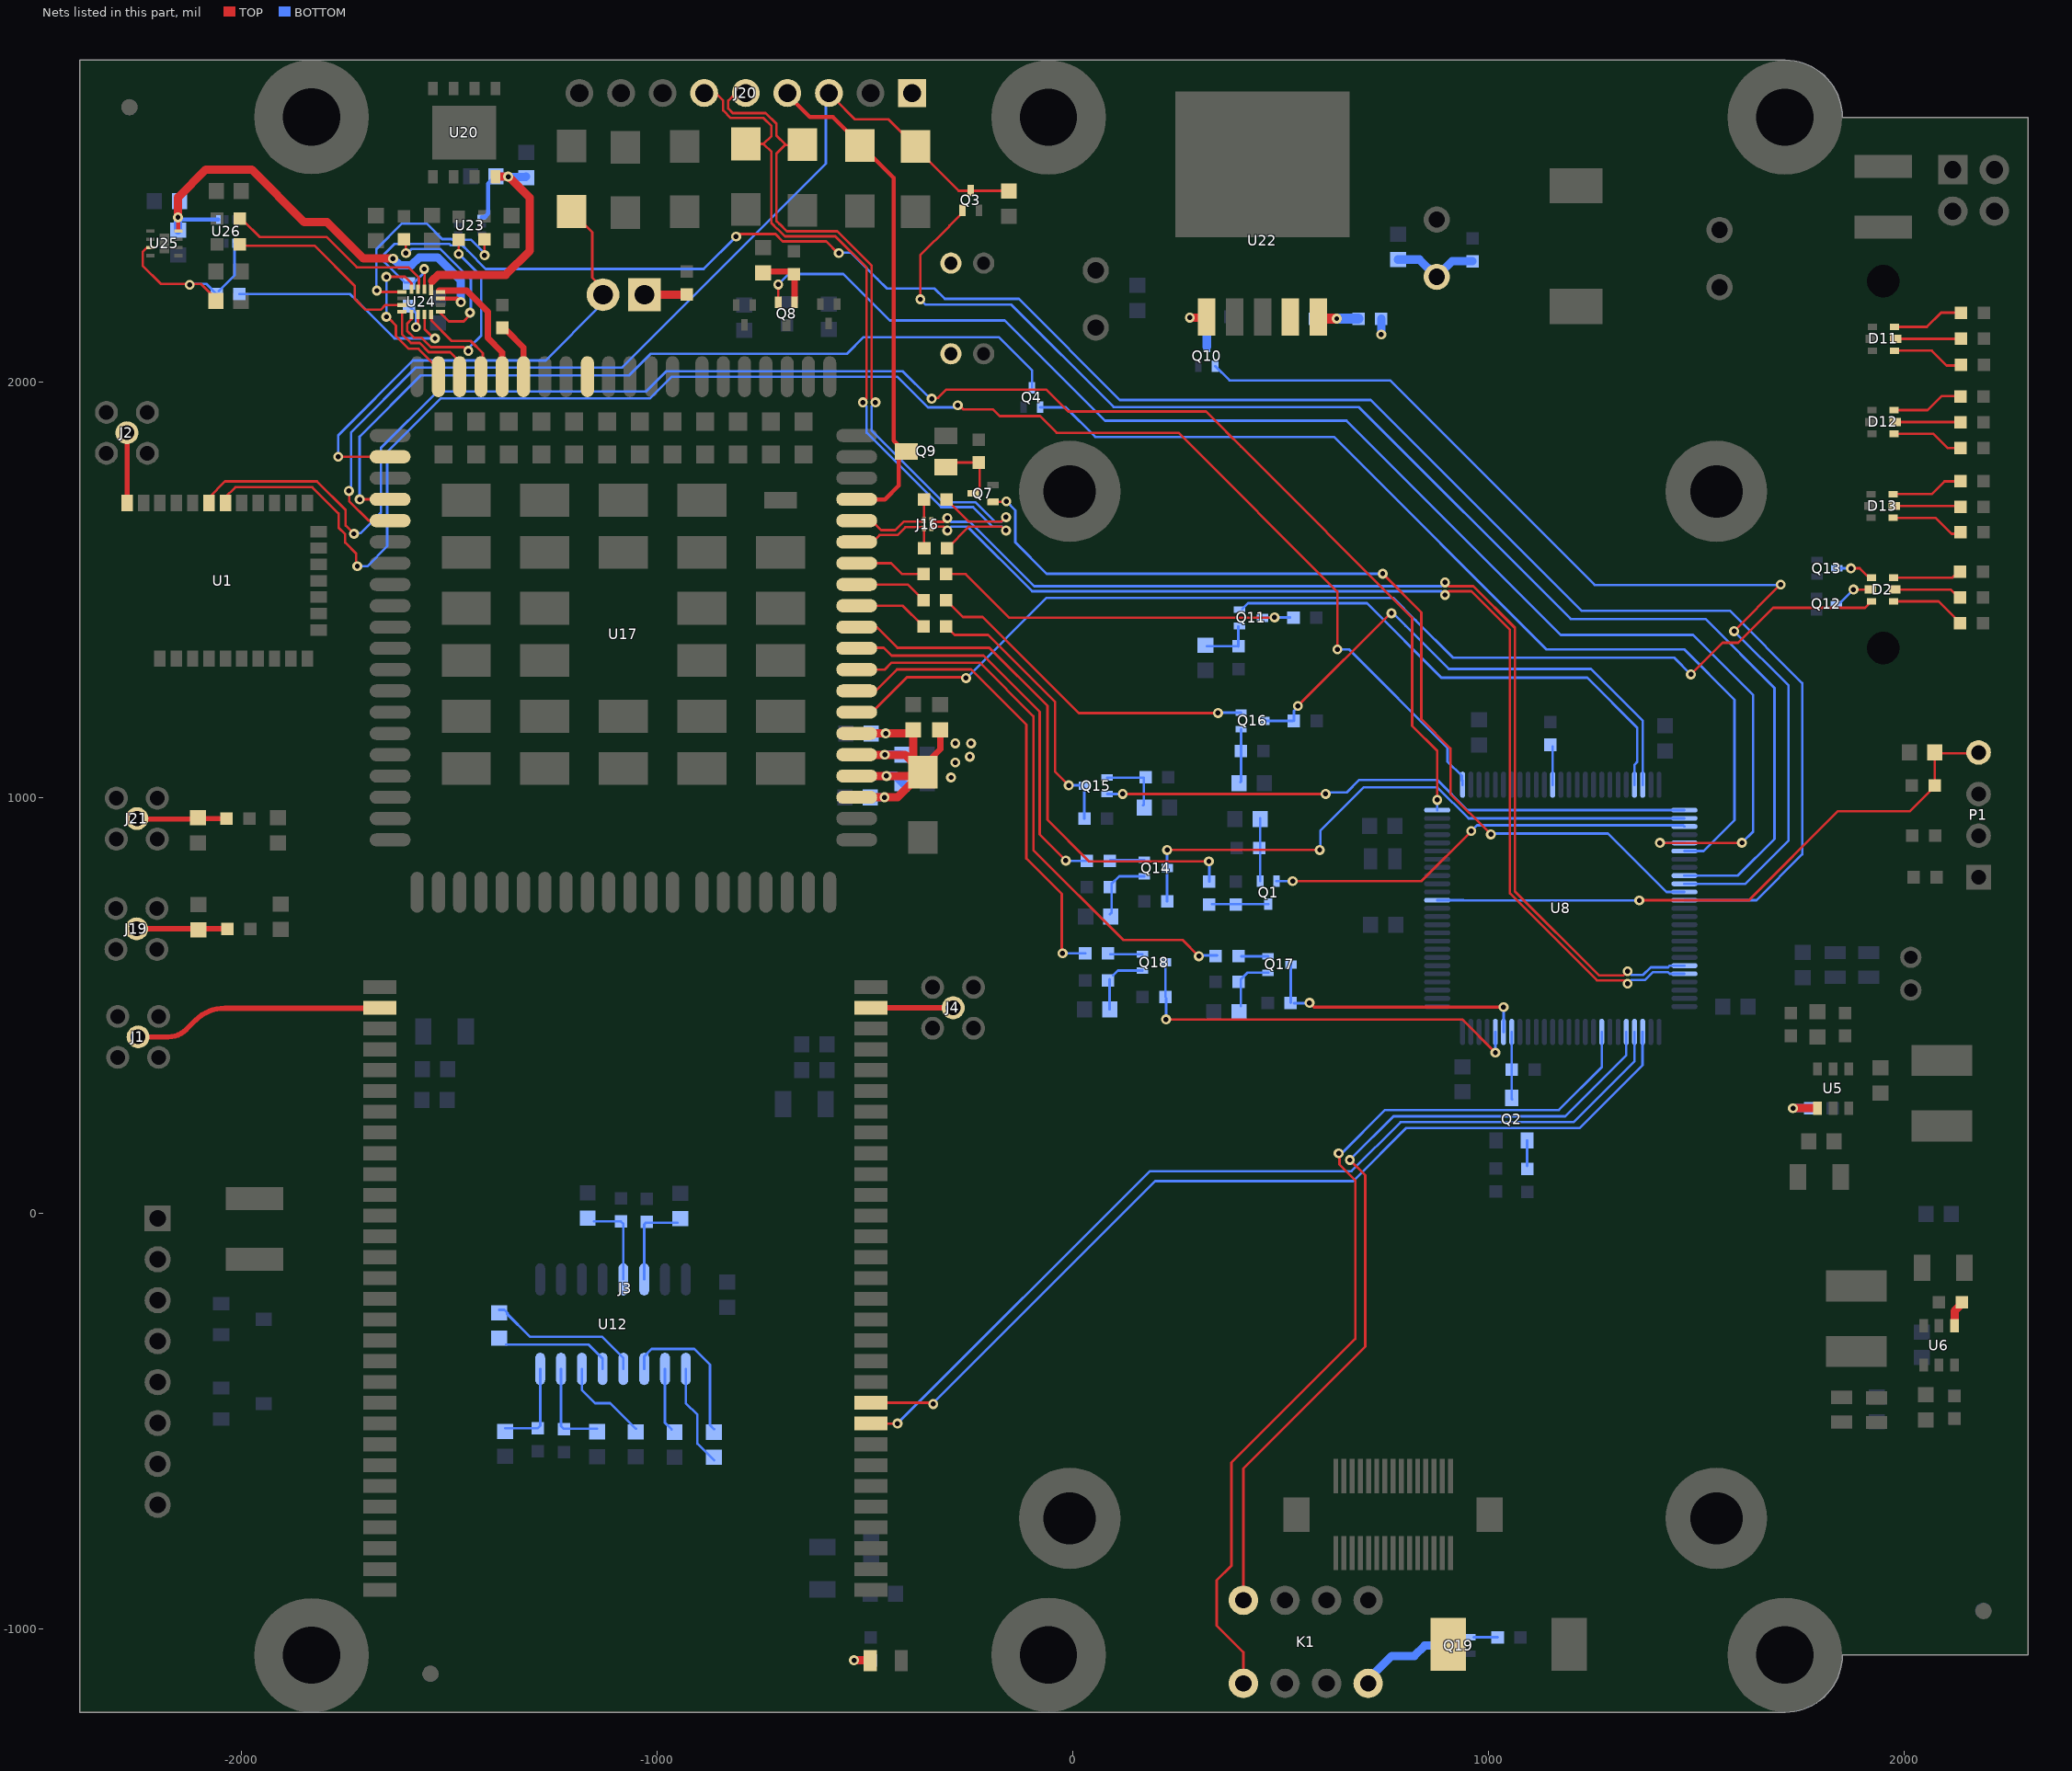
[diagram p0: the nets of this part, all layers, seen from the top]
# Altium PCB MISC84456.PcbDoc (part 4 of 5)
Units mil, origin at the board's own origin, x right, y up, seen from the top; angles counter-clockwise.
Board outline 4685.04 x 3973.82 mil, 4 copper layers (TOP, GND, POWER, BOTTOM), stack 38.4 mil thick; 219 components, 175 nets, 938 pads, 792 vias.

## Via types
v1: diameter 24, hole 12, TOP to BOTTOM, 400 vias
v2: diameter 24, hole 12, TOP to BOTTOM, tented both sides, 388 vias
v3: diameter 40, hole 20, TOP to BOTTOM, 4 vias

## Nets (pads, with @x,y where several pads share a name; then routed paths per layer and width w, separated by ;. In a path a pad name is that pad's centre, name@x,y a point inside that pad or via, vN(x,y) a via of type N, cw(c..) or ccw(c..) an arc to the next point about the centre after c; other vN are vias at no path point) (continued)
NetC52_1: C52.1 R24.2 U25.3 U26.4 | length 451.1
  TOP w6: U25.3@-2218.15,2323.71 -2226.29,2323.71 -2237,2313 -2237,2280 -2193,2236 -2097,2236 C52.1@-2071,2210
  BOTTOM w6: v2@-2118,2236 -2083.74,2236 R24.2@-2059.18,2211.44 ; R24.2@-2054,2219 -2016,2257 -2016,2313 U26.4@-2016,2334.11
  other v2: -2124,2234
NetC57_2: C57.2 Q1.2 R39.1 | length 151.1
  BOTTOM w6: Q1.2@450.32,799.56 C57.2@450.32,949 C57.2@450.32,950.69
NetC58_1: C58.1 Q8.2 R31.2 | length 144.2
  TOP w6: R31.2@-671,2263 R31.2@-669.31,2264.69
  TOP w15: C58.1@-740,2266 -675,2266 -669.31,2260.32 Q8.2@-669.31,2191.56
NetC59_2: C59.2 Q11.2 R40.1 | length 123.8
  BOTTOM w6: C59.2@322.5,1364.5 R40.1@397.69,1364.5 ; R40.1@397.69,1364 R40.1@397.69,1364.5 ; Q11.2@397.69,1412.32 R40.1@397.69,1364.5 ; R40.1@398,1364.5 R40.1@397.69,1364.5
NetC60_2: C60.2 Q15.2 R43.1 | length 155.5
  BOTTOM w6: Q15.2@82.56,1048.69 170.69,1048.69 170.69,983.69 C60.2@169,982
NetC61_1: C61.1 Q14.2 R48.2 | length 160.7
  BOTTOM w6: C61.1@89,720 93,724 93,793 111.32,811.32 Q14.2@171.44,811.32
NetC62_1: C62.1 Q16.2 R51.2 | length 127.9
  BOTTOM w6: C62.1@403,1038 404.44,1039.44 Q16.2@404.44,1165.32
NetC63_1: C63.1 Q17.2 R54.2 | length 136.8
  BOTTOM w6: C63.1@404,499 404,564 419.32,579.32 Q17.2@469.44,579.32
NetC64_1: C64.1 Q18.2 R56.2 | length 147.8
  BOTTOM w6: C64.1@88.32,491 R56.2@88.32,563.69 ; R56.2@97,573 108.32,584.32 Q18.2@167.44,584.32
NetC87_1: C87.1 U12.3 | length 370.4
  BOTTOM w6: U12.3@-1031,-373.59 -1031,-343.8 -1013,-325.8 -910.2,-325.8 -873,-363 -873,-508.6 C87.1@-863,-518.6
NetC87_2: C87.2 U12.1 | length 257.6
  BOTTOM w6: -931,-444.6 -931,-435 ; U12.1@-931,-373.59 -931,-435 ; C87.2@-863,-593.4 -903.1,-553.3 -903.1,-483.9 -931,-456 -931,-435
NetC92_1: C92.1 U12.2 | length 226.6
  BOTTOM w6: -981,-495.6 -981,-421 ; U12.2@-981,-373.59 -981,-421 ; C92.1@-965,-519 -981,-503 -981,-421
NetC93_1: C93.1 U12.5 | length 270.7
  BOTTOM w6: C93.1@-1363,-315 -1165,-315 -1131,-349 U12.5@-1131,-373.59
NetC93_2: C93.2 U12.4 | length 373.7
  BOTTOM w6: C93.2@-1380,-231.6 -1367.4,-231.6 -1359.5,-239.5 ; C93.2@-1361,-241 -1306,-296 -1133,-296 -1081,-348 U12.4@-1081,-373.59
NetC94_2: C94.2 R59.2 U12.14 | length 213.9
  BOTTOM w6: U12.14@-1031,-158.2 -1031,-26 -1027,-22 C94.2@-951,-22
NetC95_2: C95.2 R60.2 U12.13 | length 206.7
  BOTTOM w6: C95.2@-1152,-19 -1087,-19 -1081,-25 U12.13@-1081,-158.2
NetC96_1: C96.1 U12.6 | length 219.2
  BOTTOM w6: U12.6@-1181,-373.59 -1181,-424 -1149,-456 -1112.6,-456 C96.1@-1051,-517.6
NetC97_2: C97.2 J19.1 R62.2 | length 207.5
  TOP w12.5: J19.1@-2240,686 -2240,685 R62.2@-2033.5,685
NetC99_1: C99.1 R63.2 U12.8 | length 223.3
  BOTTOM w6: C99.1@-1365,-516.5 -1287.1,-516.5 -1281,-510.4 U12.8@-1281,-373.59
NetC100_1: C100.1 R61.2 U12.7 | length 227.3
  BOTTOM w6: U12.7@-1231,-373.59 -1231,-511.4 -1224.9,-517.5 C100.1@-1144,-517.5
NetC102_2: C102.2 J21.1 R64.2 | length 208.5
  TOP w12.5: J21.1@-2243,949 -2101,949 -2101,950 R64.2@-2035.5,950
NetD1_1: D1.1 K1.8 Q19.3 | length 214.9
  BOTTOM w20: K1.8@716,-1115 767,-1064 821,-1064 846,-1039 Q19.3@899.44,-1039
NetD2_2: D2.2 R1.2 | length 172.3
  TOP w6: D2.2@1973.57,1472.46 2081.54,1472.46 R1.2@2127,1427
NetD2_3: D2.3 Q12.3 | length 84.3
  TOP w6: v1(1877,1501) D2.3@1917.47,1501
  BOTTOM w6: Q12.3@1846,1470 v1(1877,1501)
NetD2_4: D2.4 R2.2 | length 151.4
  TOP w6: D2.4@1976.53,1501 2111,1501 R2.2@2123,1489
NetD2_5: D2.5 Q13.3 | length 85.1
  TOP w6: v1(1871,1552) 1892,1552 D2.5@1913,1531
  BOTTOM w6: Q13.3@1836.62,1552 v1(1871,1552)
NetD2_6: D2.6 R3.2 | length 158.2
  TOP w6: D2.6@1973.57,1529.54 2115.54,1529.54 R3.2@2127,1541
NetD7_1: D7.1 R18.2 | length 79.2
  TOP w20: v2(-526.5,-1074.5) -488.5,-1074.5 D7.1@-488,-1074
  BOTTOM w20: v2(-526.5,-1074.5) R18.2@-486,-1074.5
NetD11_2: D11.2 R75.2 | length 175.1
  TOP w6: D11.2@1975.57,2075.46 2065.54,2075.46 2101,2040 R75.2@2136,2040
NetD11_4: D11.4 R76.2 | length 161.5
  TOP w6: D11.4@1978.53,2104 R76.2@2135.5,2104 R76.2@2140,2104
NetD11_6: D11.6 R81.2 | length 173.7
  TOP w6: D11.6@1975.57,2132.54 2053.54,2132.54 2088,2167 R81.2@2135,2167
NetD12_2: D12.2 R82.2 | length 172.7
  TOP w6: D12.2@1974.57,1875.46 2069.54,1875.46 2104,1841 R82.2@2133,1841
NetD12_4: D12.4 R86.2 | length 151.5
  TOP w6: D12.4@1977.53,1904 R86.2@2129,1904
NetD12_6: D12.6 R92.2 | length 170.3
  TOP w6: D12.6@1974.57,1932.54 2055.54,1932.54 2089,1966 R92.2@2131,1966
NetD13_2: D13.2 R85.2 | length 180.4
  TOP w6: D13.2@1972.57,1673.46 2074.54,1673.46 2113,1635 R85.2@2137,1635
NetD13_4: D13.4 R91.2 | length 157.5
  TOP w6: D13.4@1975.53,1702 R91.2@2133,1702
NetD13_6: D13.6 R94.2 | length 173
  TOP w6: D13.6@1972.57,1730.54 2065.54,1730.54 2096,1761 R94.2@2133,1761
NetJ1_1: J1.1 J3.2 | length 614
  TOP w12.5: J1.1@-2248,425 -2175.46,425 ccw(c-2175.46,486.46) -2132,443 -2110.29,464.71 cw(c-2039.58,394) -2039.58,494 J3.2@-1673,494 ; J3.2@-1678.58,495 J3.2@-1666.55,495 ccw(c-1671.38,490.17) J3.2@-1671.38,497
NetJ2_1: J2.1 U1.29 | length 154.3
  TOP w12.5: U1.29@-2274.31,1709.01 J2.1@-2274.31,1863.32
NetJ3_59: J3.59 J4.1 | length 175
  TOP w12.5: J3.59@-461,497 -461,495 J4.1@-288,495
NetJ16_2: J16.2 R33.2 U17.69 | length 221.7
  TOP w6: U17.69@-519.98,1615.44 -481.56,1615.44 -465,1632 -422,1632 -403,1651 J16.2@-360,1651 ; R33.2@-357.86,1601.14 J16.2@-357.86,1648.16
NetJ16_3: J16.3 R34.2 U17.70 | length 219.7
  TOP w6: U17.70@-519.98,1666.62 -483.62,1666.62 -461,1644 -426.97,1644 -406.92,1664.05 J16.3@-361,1664.05 ; J16.3@-357.86,1667.84 R34.2@-357.86,1710.86
NetJ26_1: J26.1 R77.2 | length 77.5
  TOP w20: J26.1@-1006.5,2210.5 R77.2@-929,2210.5
NetQ1_3: Q1.3 R26.1 R41.2 | length 135.4
  BOTTOM w6: R26.1@334.56,744.44 Q1.3@470,744.44
NetQ2_1: Q2.1 R37.1 | length 61.2
  BOTTOM w6: R37.1@1092.4,114.6 Q2.1@1092.4,175.82
NetQ2_3: Q2.3 R36.2 U8.94 | length 162.2
  BOTTOM w6: U8.94@1055.24,436.88 1055.24,275.76 Q2.3@1056,275
NetQ7_3: Q7.3 Q9.1 R29.2 | length 172
  TOP w6: Q9.1@-298,1806 -297.62,1806.38 R29.2@-222,1806.38 ; Q7.3@-230,1737 -224,1743 -224,1781 ; -224,1750.62 -224,1781 ; R29.2@-224,1800 -224,1781
NetQ10_3: Q10.3 R65.1 U22.1 | length 132.4
  TOP w20: v2(281,2155) U22.1@303,2155
  BOTTOM w20: v2(281,2155) 322,2155 Q10.3@322,2085.62
NetQ11_3: Q11.3 R32.1 R44.2 | length 894
  TOP w6: R32.1@-304.5,1538 -258,1538 -153,1433 v1@480,1433 ; v1@482.5,1430.5 v1@485,1433
  BOTTOM w6: Q11.3@455.56,1433 v1@481,1433 ; v1(485,1434) R44.2@522,1434
NetQ14_1: Q14.1 R47.1 | length 81.8
  BOTTOM w6: R47.1@89.69,850.69 Q14.1@171.44,850.69
NetQ15_3: Q15.3 R27.1 R45.2 | length 665.1
  TOP w6: R27.1@-304.5,1412 -284.5,1392 -204,1392 -43,1231 -43,1063 v1(-10,1030)
  BOTTOM w6: v1(-10,1030) 24,1030 Q15.3@24,1024.5 ; R45.2@27.5,950 Q15.3@27.5,1024.5
NetQ16_1: Q16.1 R28.1 | length 815.9
  TOP w6: R28.1@-304.5,1475 -264.5,1435 -217,1435 14,1204 v1(349,1204)
  BOTTOM w6: v1(349,1204) v1@350,1205 ; v1@355.69,1204.69 Q16.1@404.44,1204.69
NetQ17_1: Q17.1 R50.1 | length 64.8
  BOTTOM w6: R50.1@404.69,618.69 Q17.1@469.44,618.69
NetQ18_1: Q18.1 R52.1 | length 77.8
  BOTTOM w6: R52.1@89.69,623.69 Q18.1@167.44,623.69
NetQ19_2: Q19.2 R57.1 | length 57.5
  BOTTOM w6: Q19.2@964,-1019 R57.1@1021.5,-1019
NetR12_1: R12.1 U5.4 | length 103
  TOP w20: v1(1731.6,253.4) U5.4@1790.6,253.4
  BOTTOM w20: v1(1731.6,253.4) R12.1@1775.6,253.4
NetR19_1: R19.1 U6.4 | length 57.2
  TOP w20: U6.4@2120.4,-269.76 2120.4,-234.6 R19.1@2136,-219
NetR22_2: R22.2 U24.10 | length 83.5
  TOP w6: v2(-1580,2132) -1574.87,2137.13 U24.10@-1574.87,2162.44
  BOTTOM w6: R22.2@-1592,2178 -1580,2166 v2(-1580,2132)
NetR26_2: R26.2 U17.65 | length 1283.5
  TOP w6: U17.65@-519.98,1410.72 -471.72,1410.72 -422,1361 -346,1361 -201,1361 -61,1221 -61,947 39,847 v1(327,847)
  BOTTOM w6: R26.2@328,798.5 v1@328,841
NetR27_2: R27.2 U17.66 | length 176
  TOP w6: U17.66@-519.98,1461.9 -408.9,1461.9 R27.2@-363,1416
NetR28_2: R28.2 U17.67 | length 166.8
  TOP w6: U17.67@-519.98,1513.08 -397.08,1513.08 R28.2@-366,1482
NetR32_2: R32.2 U17.68 | length 169.9
  TOP w6: U17.68@-519.98,1564.26 -437.26,1564.26 -411,1538 R32.2@-361,1538
NetR47_2: R47.2 U17.64 | length 933.4
  TOP w6: U17.64@-519.98,1359.54 U17.64@-500,1359.54 ; U17.64@-500,1359 U17.64@-487,1359 ; U17.64@-487,1361 -455,1361 -436,1342 -215,1342 -80,1207 -80,912 v1(-17,849)
  BOTTOM w6: v1@-12,848 R47.2@33.5,848
NetR50_2: R50.2 U17.63 | length 1355.8
  TOP w6: U17.63@-519.98,1308.35 -452.65,1308.35 -436,1325 -224,1325 -95,1196 -95,874 121,658 264,658 v1(303,619)
  BOTTOM w6: v1(303,619) 305,621 R50.2@347,621
NetR52_2: R52.2 U17.62 | length 1121.2
  TOP w6: U17.62@-519.98,1257.17 -474.83,1257.17 -423,1309 -245,1309 -112,1176 -112,854 -27,769 v1@-27,629
  BOTTOM w6: v1(-25,626) R52.2@29.5,626
NetR66_1: R66.1 R68.2 U22.5 | length 143.2
  TOP w25: U22.5@588,2153 588.5,2152.5 v1(634.5,2152.5)
  BOTTOM w25: R68.2@590,2152.5 v1(634.5,2152.5) R66.1@686.5,2152.5
NRST: C1.2 P1.4 R35.1 U8.14 | length 1488.2
  TOP w6: v1@1356,756 1358.19,753.81 1557,753.81 1625.81,753.81 1840,968 2013,968 R35.1@2071,1026 ; R35.1@2072.5,1030 2072.5,1103.5 2076,1107 P1.4@2172,1107
  BOTTOM w6: U8.14@876.11,753.81 938.81,753.81 ; 939.63,753 v1(1362,753)
ON/OFF_MCU: Q3.1 U8.59 | length 3302.4
  TOP w6: v1@-367,2210 -367,2305 -297,2375 -297,2376 -266,2407 Q3.1@-266,2413.38
  BOTTOM w6: v1(-367,2199) -354,2186 -148,2186 98,1940 687,1940 1197,1430 1521,1430 1687,1264 1687,901 1598.86,812.86 U8.59@1470.59,812.86
PB2_BOOT1: R4.2 U8.37 | length 92
  BOTTOM w6: U8.37@1153.67,1031.36 R4.2@1153.67,1123.33
PWRKEY: C32.1 D17.2 J20.3 Q3.3 U17.21 | length 2330.4
  TOP w6: v2@-1740,1733 -1740,1712.91 -1693.71,1666.62 U17.21@-1642.02,1666.62 ; J20.3@-573,2681 -524,2632 -443.26,2632 D17.2@-378,2566.74 ; D17.2@-351,2536 -298,2483 -275,2460 -159,2460 C32.1@-157,2462
  BOTTOM w6: v2@-1743,1735 v2@-1741,1737 ; v2@-1741,1735 v2@-1741,1737 ; v2(-1741,1738) v2@-1741,1737 ; J20.3@-594,2690 -594,2525 -1084,2035 -1580,2035 -1736.2,1878.8 -1736.2,1797 -1736.2,1756 -1736.2,1741.8 v2@-1741,1737
RESET_MCU: Q4.1 U8.56 | length 2402.4
  BOTTOM w6: Q4.1@-79,1939.38 -17.38,1939.38 54,1868 573,1868 628,1868 1139,1357 1470,1357 1591,1236 1591,946 1516.92,871.92 U8.56@1470.59,871.92
RESET_N: Q4.3 U17.20 | length 2014.6
  TOP w6: v2(-1715.2,1717.8) U17.20@-1642.02,1717.8
  BOTTOM w6: v2(-1715.2,1717.8) -1715.2,1868.8 -1568,2016 -1067,2016 -1015,2068 -543,2068 -503,2108 -178,2108 -98,2028 Q4.3@-98,1987
SIM_SEL: R22.1 U8.62 U24.2 | length 5006.5
  TOP w6: -1559.69,2251.18 -1559.69,2224.13 U24.2@-1559.13,2223.56 ; -1559.13,2251.74 v2@-1559.13,2269.13 ; v2(-810,2350) -804,2356 -715.21,2356 -697.71,2338.5 -593.5,2338.5 v2@-564,2309
  BOTTOM w6: R22.1@-1591,2239.5 -1607.2,2239.5 -1656,2288.3 -1656,2308 -1632,2332 -1499.07,2332 -1496.07,2329 -1468.3,2329 -1456,2316.7 -1456,2316 -1412,2272 -888,2272 v2(-810,2350) v2@-809,2351 ; R22.1@-1584,2239.5 -1559,2264.5 v2@-1559,2271 ; v2@-557,2311 -533,2311 -470,2248 ; -530,2308 -470,2248 ; -165,2200 -231,2200 ; U8.62@1470.59,753.81 1643.81,753.81 1754,864 1754,1276 1580,1450 1223,1450 716,1957 112.97,1957 -130.03,2200 -231,2200 ; -470,2248 -447,2225 -333,2225 -308,2200 -231,2200
  other v2: -1560,2272 -563,2310
SIMA_CLK: R15.1 U24.9 | length 511.7
  TOP w6: U24.9@-1590.62,2162.44 -1590.62,2151.08 -1601,2140.7 -1601,2123 -1585,2107 -1567.06,2107 -1544.06,2084 -1528,2084 -1525.3,2084 -1465,2084 v2@-1460,2079 ; v2(-1477,2308) R15.1@-1477,2342.5 ; v2@-1459.5,2081.5 v2@-1455,2077 ; v2@-1458,2077 -1457,2078 v2(-1454,2075)
  BOTTOM w6: v2(-1477,2308) -1423,2254 -1423,2112 v2@-1454,2081
SIMA_DATA: R16.1 U24.13 | length 403
  TOP w6: R16.1@-1604,2343.5 v2(-1604,2310) v2@-1601,2307 ; U24.13@-1520.59,2169.38 -1520.59,2165.59 -1501,2146 -1465,2146 v2@-1453,2158
  BOTTOM w6: v2@-1603,2308 -1591,2320 -1521.13,2320 -1448,2246.87 -1448,2163 v2@-1452,2159 ; v2@-1448,2158 v2@-1448,2159
  other v2: -1450,2167
SIMA_RST: R14.1 U24.5 | length 509.3
  TOP w6: v2@-1674,2216.62 U24.5@-1613.41,2216.62 ; v2(-1415,2305) R14.1@-1415,2343.5
  BOTTOM w6: v2@-1675,2228 -1675,2320 -1614,2381 -1554,2381 -1517,2344 -1494.1,2344 -1492.1,2342 -1447,2342 v2@-1415,2310 ; v2@-1417.5,2307.5 v2(-1415,2305)
  other v2: -1674,2220
SIMA_VDD: C24.1 C34.1 U20.8 U23.1 U24.1 | length 702.6
  TOP w10: U24.1@-1543.38,2221.59 -1543.38,2239.62 -1538,2245
  TOP w20: -1540.69,2243.31 -1526,2258 -1364,2258 -1306,2316 -1306,2443 -1357,2494 v2(-1358,2494) U20.8@-1386,2494
  BOTTOM w10: U23.1@-1421.56,2396.69 -1414.31,2396.69 -1406,2405 -1406,2477 C34.1@-1393,2490
  BOTTOM w20: C34.1@-1389,2494 v2(-1358,2494) ; v2@-1358,2493 -1316.5,2493 C24.1@-1315,2494.5
SIMB_CLK: R23.1 U24.7 | length 471.1
  TOP w6: R23.1@-1998,2328 -1824,2328 -1727,2231 -1727,2200 -1701,2174 -1665,2174 -1653.87,2185.13 U24.7@-1613.41,2185.13
SIMB_DATA: R24.1 U24.11 | length 580.2
  TOP w6: U24.11@-1559.13,2162.44 -1559,2162.31 -1559,2127 v2@-1538,2106
  BOTTOM w6: R24.1@-2004.18,2211.44 -1738.14,2211.44 -1722,2195.3 ; -1722,2197 -1722,2195.3 ; v2@-1538,2105 -1631.7,2105 -1722,2195.3 ; v2(-1534,2105) v2@-1534,2108
SIMB_RST: R21.1 U24.3 | length 502.3
  TOP w6: R21.1@-1994,2387 -1956,2349 -1795,2349 -1722,2276 -1598,2276 -1573,2251 U24.3@-1573,2226
SIMB_VDD: C45.1 C49.1 U24.15 U25.8 U26.1 | length 1158.6
  TOP w10: v2(-2152.18,2396.19) -2152.18,2365.19 U25.8@-2152,2365 ; U24.15@-1520.59,2200.87 -1480.87,2200.87 v2(-1472,2192)
  TOP w20: v2@-2152,2404 -2152,2444 -2085,2511 -1975,2511 -1848.5,2384.5 -1793.5,2384.5 -1706,2297 v2(-1635,2297)
  BOTTOM w10: v2@-2144,2391 U26.1@-2055.37,2391
  BOTTOM w20: C49.1@-2152.18,2365.19 v2(-2152.18,2396.19) C45.1@-2152.18,2425.56 ; v2(-1635,2297) -1619,2281 -1590.6,2281 -1571.6,2300 -1528,2300 -1472,2244 v2(-1472,2192)
SLEEP_STATUS: Q8.1 U8.55 | length 3597.1
  TOP w6: Q8.1@-708.68,2191.56 v2(-708.68,2234.69) ; v1(1411.6,891.6) v1@1613.6,891.6
  BOTTOM w6: v2(-708.68,2234.69) -683.37,2260 -552,2260 -440,2148 -354,2148 ; -202,2148 -354,2148 ; v1(1411.6,891.6) U8.55@1470.59,891.6 ; v1(1609,892) 1636,919 1636,1247 1491,1392 1173,1392 658,1907 77,1907 -164,2148 -354,2148
STATUS: D2.1 U17.61 | length 2707.9
  TOP w6: U17.61@-519.98,1205.99 -483.01,1205.99 -399,1290 v1@-256,1290 ; v1(1486,1297) 1562,1373 1600,1373 1684,1457 1904.97,1457 D2.1@1920.42,1472.46
  BOTTOM w6: v1(-257,1288) -257,1287 -63,1481 770,1481 825,1426 ; 824,1427 825,1426 ; v1(1486,1297) 1446,1337 914,1337 825,1426
UART2_RXD: U1.23 U8.26 | length 3951.4
  TOP w6: U1.23@-2039,1722 -2014,1747 -1829,1747 -1766,1684 -1766,1650 -1750,1634 -1750,1614 -1724,1588 -1724,1560 v1(-1721,1557) ; v1@-272,1943 -263,1934 -192,1934 -176,1918 -79,1918 -39,1878 254,1878 636,1496 v1(636,1357)
  BOTTOM w6: v1(-1721,1557) -1697,1557 -1649,1605 -1649,1832 -1520,1961 -1017,1961 -965,2013 -422.3,2013 -354.15,1944.85 -348.3,1939 -283,1939 v1@-280,1942 ; v1@-279.5,1941.5 v1(-277,1944) ; v1(636,1357) 664,1357 901,1120 901,1087 935,1053 U8.26@935,1041 ; U8.26@937.13,1031.36 U8.26@937.13,1041
UART2_TXD: U1.24 U8.25 | length 4047.8
  TOP w6: U1.24@-2077.46,1709.01 -2077.46,1722.54 -2039,1761 -1818,1761 -1749,1692 -1749,1655 v1(-1729,1635) ; v1@-344,1962 -324,1962 -304,1982 -64,1982 -11,1929 320,1929 404,1845 ; 369,1880 404,1845 ; v1(876.11,994.89) 876.11,1112.89 816,1173 816,1433 404,1845
  BOTTOM w6: v1@-1727.56,1636.44 -1713.56,1636.44 -1664,1686 -1664,1842 -1529,1977 -1027,1977 -978,2026 -409,2026 v1@-344,1961 ; U8.25@876.11,970.34 v1(876.11,994.89)
  other v1: -339.6,1960
UART3_CTS: Q14.3 R46.1 U8.52 | length 1479.4
  TOP w6: v1(226.56,874.56) v1(593.44,874.56)
  BOTTOM w6: R46.1@226.5,751 Q14.3@226.5,827.5 ; Q14.3@226.56,831 v1(226.56,874.56) ; v1@595,878 595,921 699,1025 877,1025 951.34,950.66 U8.52@1470.59,950.66
UART3_DCD: Q17.3 R53.1 U8.95 | length 662.5
  TOP w7: v1(569,507) 579.45,496.55 v1(1035.55,496.55)
  BOTTOM w7: R53.1@523.5,507 Q17.3@523.5,601.5 ; R53.1@532,506 568,506 v1(569,507) ; U8.95@1035.55,436.88 v1(1035.55,496.55)
UART3_DTR: Q15.1 U8.51 | length 1427.2
  TOP w6: v1(119.69,1009.32) v1(607.69,1009.32)
  BOTTOM w6: Q15.1@82.56,1009.32 v1(119.69,1009.32) ; v1@611,1013 659,1013 689,1043 876,1043 948.66,970.34 U8.51@1470.59,970.34
UART3_RI: Q18.3 R55.1 U8.96 | length 1006.6
  TOP w6: v1(224,467) 936,467 v1(1015.87,387.13)
  BOTTOM w6: R55.1@222.5,521 Q18.3@222.5,602.5 ; v1(224,467) 224,516 R55.1@225,517 ; v1(1015.87,387.13) U8.96@1015.87,436.88
UART3_RTS: Q1.1 U8.53 | length 1037.8
  TOP w6: v1(528.44,799.56) 837.56,799.56 v1(958,920)
  BOTTOM w6: Q1.1@489.69,799.56 v1(528.44,799.56) ; v1(958,920) 972,934 1467.57,934 U8.53@1470.59,930.97
UART3_RXD: Q16.3 R49.1 U8.48 | length 1316.8
  TOP w6: v1(541,1221) v1@766,1446 ; v1(766,1444) v1@766,1446 ; v1@766,1446 766,1448 770,1450 v1@766,1446
  BOTTOM w6: Q16.3@459.56,1185 R49.1@528,1185 ; R49.1@531.5,1185 531.5,1209.5 v1@540.41,1218.41 ; v1@541,1219 v1@540.41,1218.41 ; v1(541,1221) 540.57,1219.1 v1@540.41,1218.41 ; v1(766,1444) 766,1448 800,1414 ; 797,1417 800,1414 ; U8.48@1370.2,1031.36 1370.2,1185.8 1246,1310 904,1310 800,1414
UART3_TXD: Q11.1 U8.47 | length 1220
  BOTTOM w6: Q11.1@407,1454 421,1468 707,1468 886,1289 1237,1289 1357,1169 1357,1086 1350.52,1079.52 U8.47@1350.52,1031.36
UART4_RXD: J3.39 U8.79 | length 2249.9
  TOP w6: J3.39@-466,-505 v2(-422,-505)
  BOTTOM w6: U8.79@1350.52,436.88 1350.52,366.52 1204,220 981,220 788,220 670,102 185,102 v2@-421,-504 ; v2@-421,-504 -421,-505 v2(-422,-505) v2@-421,-504
UART4_TXD: J3.40 U8.78 | length 2273.7
  TOP w6: J3.40@-485.45,-455 v2@-345,-455
  BOTTOM w6: v2@-345,-457 -345,-455 -335,-455 198,78 674,78 802,206 962,206 1219,206 1370,357 U8.78@1370,436.88
  other v2: -336,-458
UART5_RXD: K1.5 U8.83 | length 2280.1
  TOP w6: K1.5@410,-1130 410,-1055 346,-991 346,-882 381,-847 381,-599 679,-301 679,80 641,118 v1@641,145 ; v1@632,145 v1(639,145)
  BOTTOM w6: v1@634,146 648,146 751,249 1169,249 1271.78,351.78 U8.83@1271.78,436.88 ; v1@634,147 632,145 v1(639,145)
UART5_TXD: K1.4 U8.80 | length 2016.6
  TOP w6: K1.4@410,-930 410,-613 703,-320 703,92 v1(666,129)
  BOTTOM w6: v1@669,132 771,234 964,234 1184,234 1330.83,380.83 U8.80@1330.83,436.88
USB-DM2: J16.4 U8.70 | length 2673.3
  TOP w6: J16.4@-339,1665 -338.05,1664.05 -322.05,1664.05 -322,1664 ; -330,1664 -322,1664 ; v2(-302,1673) -311,1664 -322,1664 ; v1(895,1518) 904,1509 962.97,1509 1063,1408.97 1063,775 1265,573 1324,573 v1(1334,583)
  BOTTOM w6: v2(-302,1673) -293,1664 -248,1664 -93,1509 886,1509 v1(895,1518) ; v1(1334,583) 1343,574 1371.03,574 1389.51,592.48 1431.28,592.48 1435.12,596.32 U8.70@1470.59,596.32
USB-DP2: J16.1 U8.71 | length 2677.1
  TOP w6: J16.1@-338,1651.95 -316.05,1651.95 -316,1652 ; -330,1652 -316,1652 ; v2(-302,1643) -311,1652 -316,1652 ; v1(895,1488) 904,1497 958,1497 1051,1404 1051,770.03 1260.03,561 1326,561 v1(1334,553)
  BOTTOM w6: v2(-302,1643) -293,1652 -252.97,1652 -97.97,1497 886,1497 v1(895,1488) ; v1(1334,553) 1343,562 1376,562 1394.48,580.48 1431.28,580.48 1435.12,576.64 U8.71@1470.59,576.64
USB_BOOT: D24.2 J26.2 U17.115 | length 1145.1
  TOP w6: v2(-1766.83,1820.17) U17.115@-1642.02,1820.17 ; D24.2@-1206,2410.26 -1156,2360.26 -1156,2251 J26.2@-1134,2229
  BOTTOM w6: v2(-1766.83,1820.17) -1766.83,1872.17 -1587,2052 -1268,2052 J26.2@-1138,2182
USB_DM_TEST: D15.2 J20.5 R34.1 | length 1736.2
  TOP w6: J20.5@-786.75,2695.12 -810.88,2695.12 -829,2677 -829,2658 -818,2647 -739.03,2647 -713,2620.97 -713,2593 -690.74,2570.74 ; -706,2380 -713,2387 -713,2550 -693,2570 D15.2@-680,2570 ; -705.27,2380 -687.77,2362.5 -566.53,2362.5 -484,2279.97 -484,1960 ; D15.2@-680,2570.74 D15.2@-651,2570.74 D15.2@-657.74,2570.74 ; R34.1@-303.5,1717 -251,1664.5 -171.5,1664.5 v1@-162,1674
  BOTTOM w6: -484,1942 -484,1883 -312,1711 -235,1711 -188.5,1664.5 -171.5,1664.5 v1(-161,1675)
  other v2: -475,1951
USB_DP_TEST: D14.2 J20.6 R33.1 | length 1735.2
  TOP w6: J20.6@-886.75,2695.12 -859.12,2695.12 -841,2677 -841,2653.03 -822.97,2635 -744,2635 -725,2616 -725,2592 -744.26,2572.74 D14.2@-787,2572.74 ; -743,2572 -725,2554 -725,2382.03 -710.97,2368 ; -710.24,2368 -692.74,2350.5 -571.5,2350.5 -496,2275 -496,1960 ; R33.1@-302.5,1600 -250,1652.5 -171.5,1652.5 v1@-163,1644
  BOTTOM w6: -496,1942 -496,1878.03 -316.97,1699 -239.97,1699 -193.47,1652.5 -170.5,1652.5
  other v1: -161,1643
  other v2: -505,1951
USB_VBUS: D16.2 J20.4 Q9.3 U17.71 | length 1194.7
  TOP w10: J20.4@-674,2679 -632,2637 -577,2637 -431,2491 -431,1859 -402,1830 -419,1813 -419,1751 -452.2,1717.8 U17.71@-519.98,1717.8
USIM_CLK: U17.16 U24.8 | length 221.3
  TOP w6: U24.8@-1613.41,2169.38 -1613.41,2115.41 -1592,2094 -1571.03,2094 -1549.03,2072 -1498,2072 U17.16@-1474,2048
USIM_DATA: U17.15 U24.12 | length 190.1
  TOP w6: U24.12@-1543,2162 -1543,2148 -1494,2099 -1448.3,2099 -1419,2069.7 U17.15@-1419,2050
USIM_GND: U17.10
USIM_PRESENCE: R42.2 U17.13 | length 127.8
  TOP w15: R42.2@-1362,2124 -1321.16,2083.16 U17.13@-1321.16,2013.08
USIM_RST: U17.17 U24.4 | length 377.1
  TOP w6: v2(-1651,2253) -1606,2253 -1590.62,2237.62 U24.4@-1590.62,2223.56 ; v2@-1644,2152 -1628,2136 -1628,2111 -1597,2080 -1574,2080 -1525.88,2031.88 U17.17@-1525.88,2013.08
  BOTTOM w6: v2(-1651,2157) v2@-1651,2252
USIM_VDD: U17.14 U24.16 | length 308.4
  TOP w15: U24.16@-1524,2220 -1458,2220 -1407,2169 -1407,2106 -1372.34,2071.34 U17.14@-1372.34,2013.08
VBAT: C70.1 C71.1 C72.1 C73.1 C74.1 C75.1 C76.1 C77.1 C104.1 C105.1 D8.2 J20.1 R66.2 R67.2 U17.57 U17.58 U17.59 U17.60 U22.4 | length 1129.7
  TOP w15: D8.2@-349,1087 -319,1117 C74.1@-319,1163.69 ; C74.1@-320,1166 C74.1@-319.4,1166.6
  TOP w20: U17.57@-519.98,1001.27 v2(-453.27,1001.27) -421.73,1001.27 D8.2@-387,1036 ; U17.58@-519.98,1052.45 v2(-448.45,1052.45) -392.55,1052.45 D8.2@-388,1057 ; U17.59@-519.98,1103.63 v2(-452.37,1103.63) -403.63,1103.63 D8.2@-388,1088 ; U17.60@-519.98,1154.81 v2@-450,1154.81 ; v2(-450,1155) v2@-450,1154.81 ; C73.1@-384,1163.69 -384,1090 D8.2@-374,1080 ; C73.1@-382,1170 -397.19,1154.81 v2@-450,1154.81
  BOTTOM w20: C75.1@-490.5,1001 C75.1@-487.68,1001 v2@-455,1001 ; C72.1@-488.5,1155 -451,1155 v2@-450,1156 ; v2(-452.37,1103.63) -452,1104 C71.1@-415,1104 ; v2@-445,1053 -426.5,1053 C70.1@-408.5,1035 ; v1(741.5,2114.5) R66.2@741.5,2152 ; C105.1@782,2294.69 833.32,2294.69 C104.1@870,2258 ; C104.1@882,2261 911.5,2290.5 R67.2@961,2290.5
  other v2: -293,1049 -283,1085 -248,1099 -283,1131 -245,1131
VBAT_EN: Q10.1 U8.60 | length 2584.2
  TOP w6: v1(1590,1401) v1(1702,1513)
  BOTTOM w6: Q10.1@342,2038.38 376.38,2004 763,2004 1255,1512 v1@1696,1512 ; U8.60@1470.59,793.18 1617.18,793.18 1721,897 1721,1270 v1(1590,1401) v1@1588.5,1402.5
VBUS_CTRL: Q7.1 U8.61 | length 2295.7
  TOP w6: Q7.1@-192.38,1712 v1@-164,1712 ; v1@750,1534 838,1446 838,1189 908,1119 908,1009 v1@1000,917
  BOTTOM w6: v1(-160,1713) -138.61,1691.61 -138.61,1614.61 -63,1539 v1(745,1539) ; v1(1005,912) 1007,914 1287,914 1427.51,773.49 U8.61@1470.59,773.49